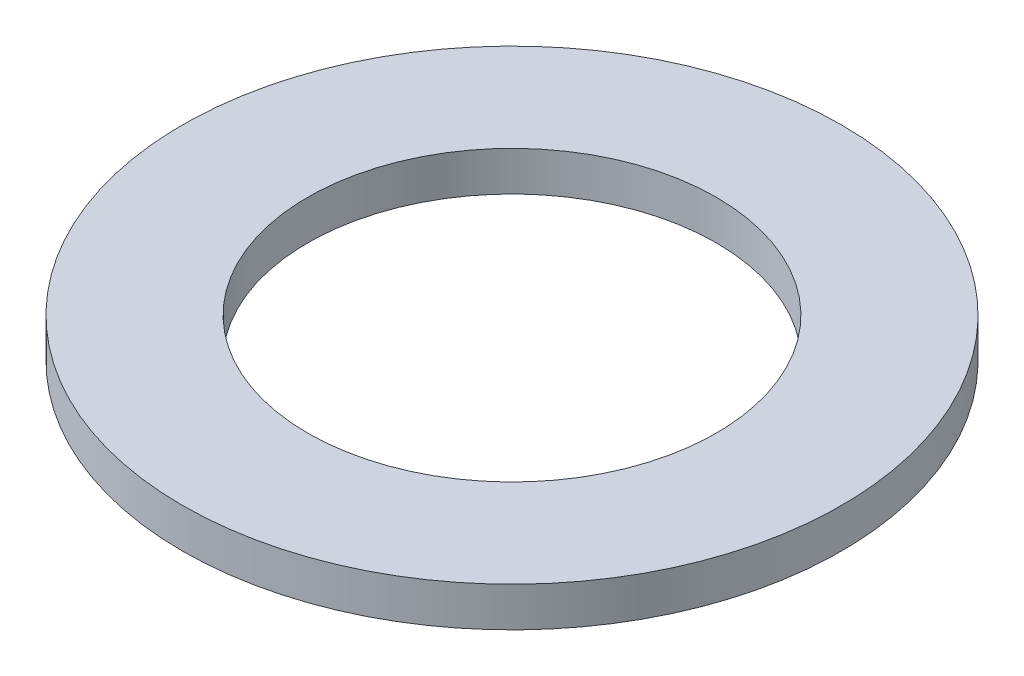
SolidWorks part; units mm, degrees
material "A3"
ref_plane "前视基准面" through (0, 0, 0) normal (0, 0, 1) x (1, 0, 0)
ref_plane "上视基准面" through (0, 0, 0) normal (0, 1, 0) x (1, 0, 0)
ref_plane "右视基准面" through (0, 0, 0) normal (1, 0, 0) x (0, 0, -1)
sketch "草图1" plane through (0, 0, 0) normal (0, 1, 0) x (1, 0, 0)
  circle A0 centre (0, 0) radius 15.5
  circle A1 centre (0, 0) radius 25
  dimension "D1" = 31
  dimension "D2" = 50
extrude "凸台-拉伸1" add sketch "草图1" along normal mid plane 3
